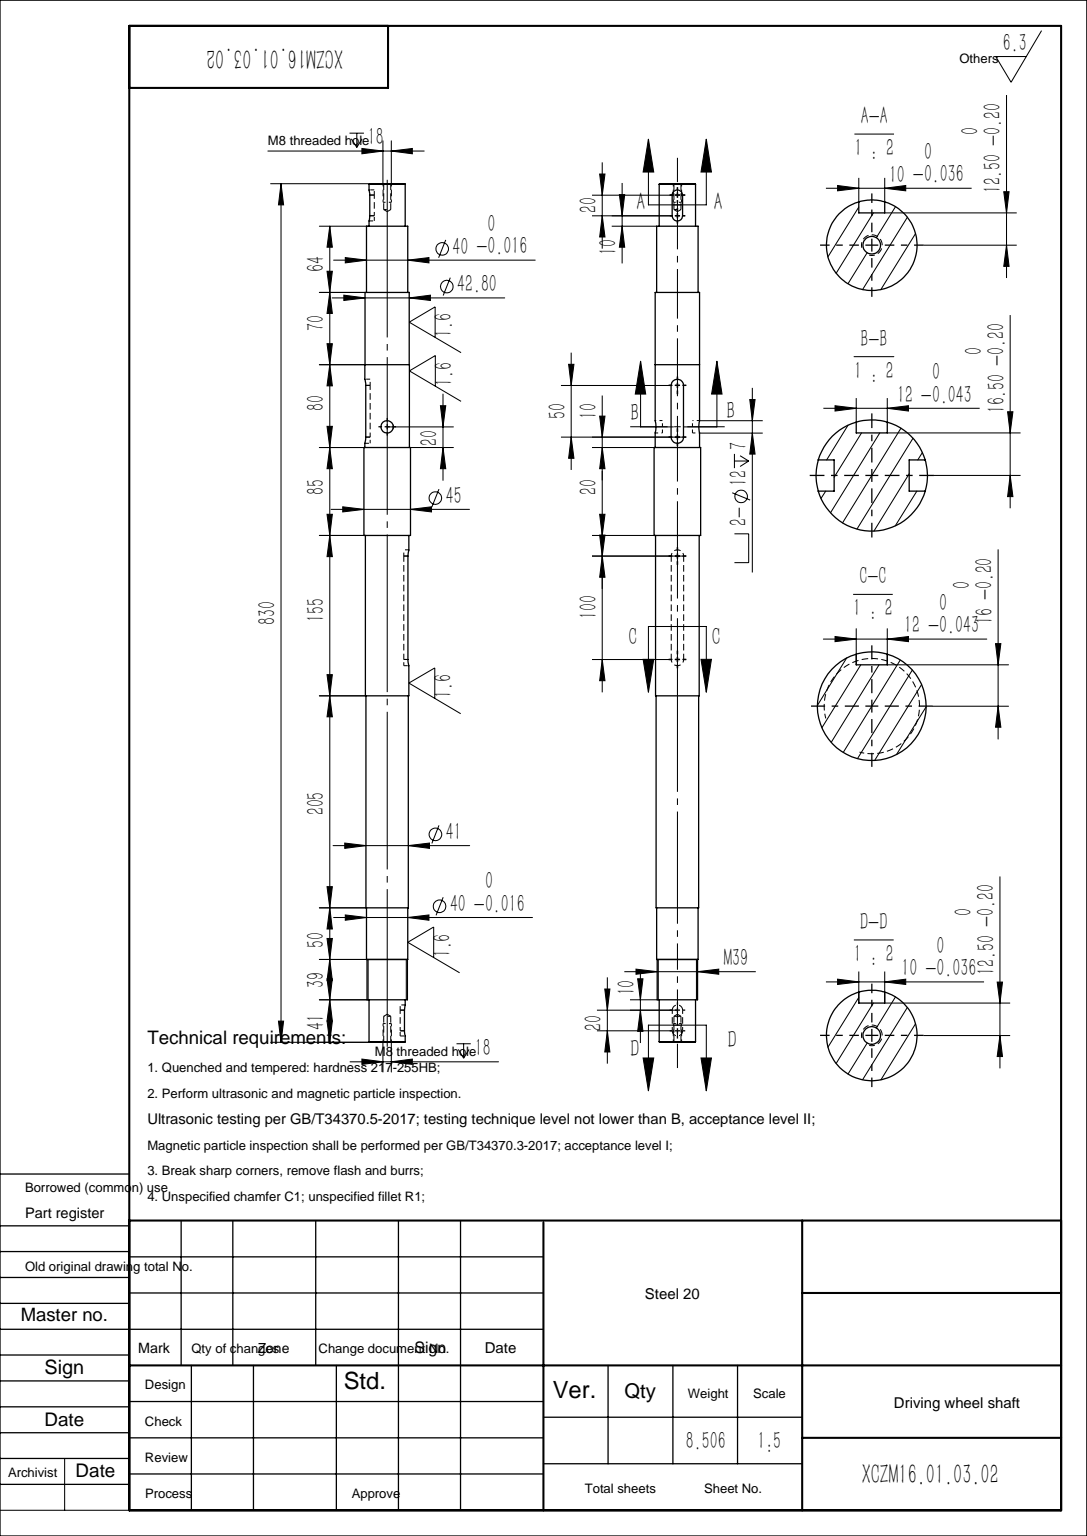
SolidWorks part; units mm, degrees
material "20 Steel"
ref_plane "Front Plane" through (0, 0, 0) normal (0, 0, 1) x (1, 0, 0)
ref_plane "Top Plane" through (0, 0, 0) normal (0, 1, 0) x (1, 0, 0)
ref_plane "Right Plane" through (0, 0, 0) normal (1, 0, 0) x (0, 0, -1)
sketch "Sketch1" plane through (0, 0, 0) normal (0, 0, 1) x (1, 0, 0)
  line L0 (0, 0) -> (0, 17.5)
  line L1 (0, 17.5) -> (41, 17.5)
  line L2 (41, 17.5) -> (41, 19.5)
  line L3 (41, 19.5) -> (80, 19.5)
  line L4 (80, 19.5) -> (80, 20)
  line L5 (80, 20) -> (130, 20)
  line L6 (130, 20) -> (130, 20.5)
  line L7 (130, 20.5) -> (335, 20.5)
  line L8 (335, 20.5) -> (335, 21)
  line L9 (335, 21) -> (490, 21)
  line L10 (490, 21) -> (490, 22.5)
  line L11 (490, 22.5) -> (575, 22.5)
  line L12 (575, 22.5) -> (575, 21.5)
  line L13 (575, 21.5) -> (655, 21.5)
  line L14 (655, 21.5) -> (655, 21.4)
  line L15 (655, 21.4) -> (725, 21.4)
  line L16 (725, 21.4) -> (725, 20)
  line L17 (725, 20) -> (789, 20)
  line L18 (789, 20) -> (789, 17.5)
  line L19 (789, 17.5) -> (830, 17.5)
  line L21 (830, 0) -> (0, 0)
  line L22 (0, 0) -> (-131.622, 0) construction
  line L26 (830, 17.5) -> (830, 0)
  point P18 (412.5, 21)
  dimension "D1" = 830
  dimension "D2" = 35
  dimension "D3" = 39
  dimension "D4" = 40
  dimension "D5" = 41
  dimension "D6" = 42
  dimension "D7" = 45
  dimension "D8" = 43
  dimension "D9" = 42.8
  dimension "D10" = 40
  dimension "D11" = 35
  dimension "D13" = 41
  dimension "D14" = 39
  dimension "D15" = 50
  dimension "D16" = 205
  dimension "D17" = 155
  dimension "D18" = 85
  dimension "D19" = 80
  dimension "D20" = 70
  dimension "D21" = 64
revolve "Revolve1" add sketch "Sketch1" angle 360 about L22
cosmetic thread "Cosmetic Thread1" parameters "D1"=39, "D2"=36.835
hole_wizard "M8 Tapped Hole1" positions "Sketch2" profile "Sketch3" tap size "M8" standard "GB"
sketch "Sketch2" plane through (0, 0, 0) normal (-1, 0, 0) x (0, 0, 1)
  point P0 (0, 0)
sketch "Sketch3" plane through (0, 0, 0) normal (0, 1, 0) x (0, 0, 1)
  line L0 (0, 0) -> (0, 27.0429)
  line L1 (0, 27.0429) -> (3.4, 25)
  line L2 (3.4, 25) -> (3.4, 0)
  line L5 (3.4, 0) -> (0, 0)
  line L10 (0, 27.0429) -> (-3.4, 25) construction
  line L11 (0, -6.35) -> (0, 107.95) construction
  dimension "螺纹孔钻头直径" = 6.8
  dimension "螺纹孔钻头深度" = 25
  dimension "导头角度" = 118
cosmetic thread "Hole Cosmetic Thread1" parameters "D1"=18, "D2"=8
hole_wizard "M8 Tapped Hole2" positions "Sketch4" profile "Sketch5" tap size "M8" standard "GB"
sketch "Sketch4" plane through (830, 0, 0) normal (1, 0, 0) x (0, 0, -1)
  point P0 (0, 0)
sketch "Sketch5" plane through (830, 0, 0) normal (0, 1, 0) x (0, 0, -1)
  line L0 (0, 0) -> (0, 27.0429)
  line L1 (0, 27.0429) -> (3.4, 25)
  line L2 (3.4, 25) -> (3.4, 0)
  line L5 (3.4, 0) -> (0, 0)
  line L10 (0, 27.0429) -> (-3.4, 25) construction
  line L11 (0, -6.35) -> (0, 107.95) construction
  dimension "螺纹孔钻头直径" = 6.8
  dimension "螺纹孔钻头深度" = 25
  dimension "导头角度" = 118
cosmetic thread "Hole Cosmetic Thread2" parameters "D1"=18, "D2"=8
ref_plane "Plane1" through (0, 0, -12.5) normal (0, 0, 1) x (1, 0, 0)
sketch "Sketch6" plane through (0, 0, -12.5) normal (0, 0, 1) x (1, 0, 0)
  line L0 (11, 0) -> (31, 0) construction
  line L2 (11, 5) -> (31, 5)
  line L3 (11, -5) -> (31, -5)
  line L4 (41, 19.5) -> (41, -19.5) construction
  line L5 (0, 17.5) -> (0, -17.5) construction
  line L6 (0, 0) -> (11, 0) construction
  arc A0 (11, 5) -> (11, -5) centre (11, 0) ccw
  arc A1 (31, -5) -> (31, 5) centre (31, 0) ccw
  point P4 (21, 0)
  dimension "D1" = 10
  dimension "D2" = 10
  dimension "D3" = 20
extrude "Cut-Extrude1" cut sketch "Sketch6" against normal up to next
ref_plane "Plane2" through (0, 0, -16) normal (0, 0, 1) x (1, 0, 0)
sketch "Sketch7" plane through (0, 0, -16) normal (0, 0, 1) x (1, 0, 0)
  line L0 (370, 0) -> (470, 0) construction
  line L1 (370, 6) -> (470, 6)
  line L2 (370, -6) -> (470, -6)
  line L3 (490, 22.5) -> (490, -22.5) construction
  arc A0 (370, 6) -> (370, -6) centre (370, 0) ccw
  arc A1 (470, -6) -> (470, 6) centre (470, 0) ccw
  point P3 (420, 0)
  dimension "D1" = 12
  dimension "D2" = 100
  dimension "D3" = 20
extrude "Cut-Extrude2" cut sketch "Sketch7" against normal up to next
ref_plane "Plane3" through (0, 0, 16.5) normal (0, 0, 1) x (1, 0, 0)
sketch "Sketch9" plane through (0, 0, 16.5) normal (0, 0, 1) x (1, 0, 0)
  line L0 (585, 0) -> (635, 0) construction
  line L1 (585, 6) -> (635, 6)
  line L2 (585, -6) -> (635, -6)
  line L3 (575, -21.5) -> (575, 21.5) construction
  arc A0 (585, 6) -> (585, -6) centre (585, 0) ccw
  arc A1 (635, -6) -> (635, 6) centre (635, 0) ccw
  point P3 (610, 0)
  dimension "D1" = 12
  dimension "D2" = 10
  dimension "D3" = 50
extrude "Cut-Extrude3" cut sketch "Sketch9" along normal up to next
ref_plane "Plane4" through (0, 0, 12.5) normal (0, 0, 1) x (1, 0, 0)
sketch "Sketch10" plane through (0, 0, 12.5) normal (0, 0, 1) x (1, 0, 0)
  line L0 (799, 0) -> (819, 0) construction
  line L1 (799, 5) -> (819, 5)
  line L2 (799, -5) -> (819, -5)
  line L3 (789, -17.5) -> (789, 17.5) construction
  arc A0 (799, 5) -> (799, -5) centre (799, 0) ccw
  arc A1 (819, -5) -> (819, 5) centre (819, 0) ccw
  point P3 (809, 0)
  dimension "D1" = 10
  dimension "D2" = 20
  dimension "D3" = 10
extrude "Cut-Extrude4" cut sketch "Sketch10" along normal up to next
sketch "Sketch11" plane through (0, 0, 0) normal (0, 1, 0) x (1, 0, 0)
  line L0 (575, -21.5) -> (575, 21.5) construction
  line L1 (575, 0) -> (595, 0) construction
  line L2 (575, -22.5) -> (575, 22.5) construction
  circle A0 centre (595, 0) radius 6
  dimension "D1" = 12
  dimension "D2" = 20
extrude "Cut-Extrude5" cut sketch "Sketch11" along normal blind 7 from offset 21.5 offset against normal yes
mirror "Mirror1" about plane through (0, 0, 0) normal (0, 1, 0) of "Cut-Extrude5"
chamfer "Chamfer1" distance 0.5 angle 45 2 edges at (830, 0, -17.5) (0, 0, -17.5)
